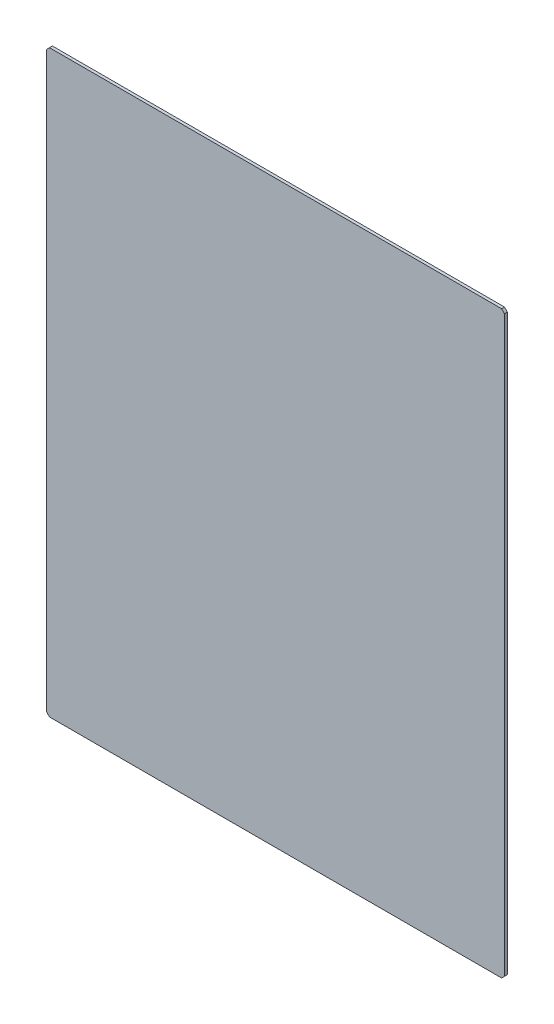
SolidWorks part; units mm, degrees
material "丙烯酸 (中高冲力)"
ref_plane "前视基准面" through (0, 0, 0) normal (0, 0, 1) x (1, 0, 0)
ref_plane "上视基准面" through (0, 0, 0) normal (0, 1, 0) x (1, 0, 0)
ref_plane "右视基准面" through (0, 0, 0) normal (1, 0, 0) x (0, 0, -1)
sketch "草图1" plane through (0, 0, 0) normal (0, 0, 1) x (1, 0, 0)
  line L0 (-395, 500) -> (395, -500) construction
  line L1 (-395, 500) -> (395, 500)
  line L2 (-395, 500) -> (-395, -500)
  line L3 (-395, -500) -> (395, -500)
  line L4 (395, 500) -> (395, -500)
  dimension "D1" = 790
  dimension "D2" = 1000
extrude "拉伸1" add sketch "草图1" along normal blind 5
chamfer "倒角1" distance 5 angle 45 4 edges at (-395, -500, 2.5) (395, -500, 2.5) (395, 500, 2.5) (-395, 500, 2.5)
